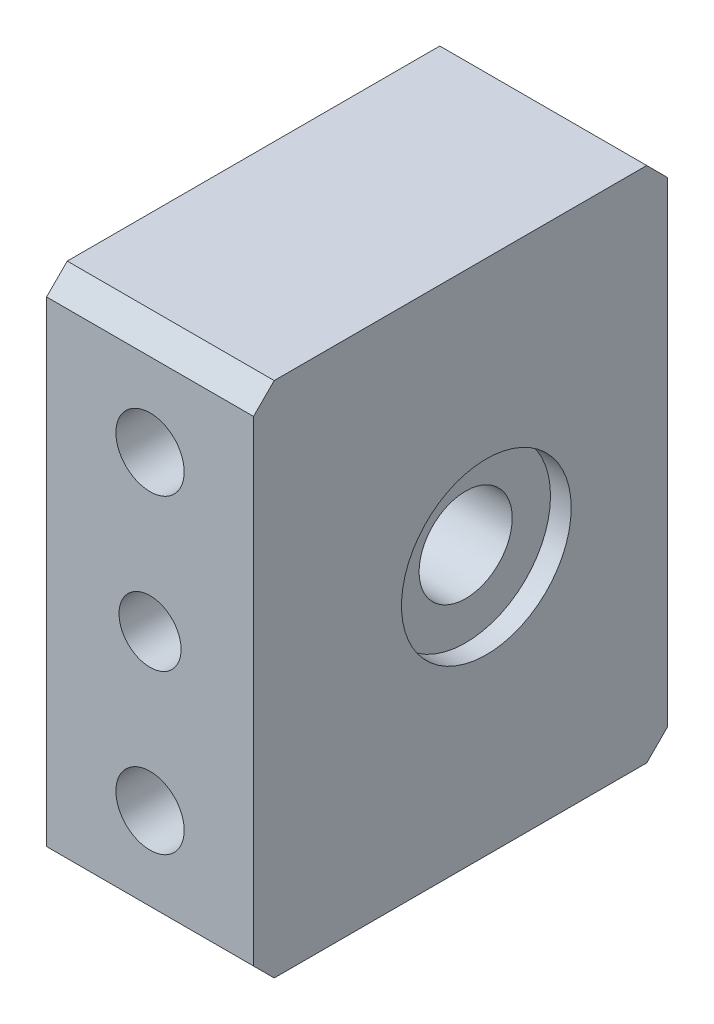
SolidWorks part; units mm, degrees
material "A6061 T6"
ref_plane "前视基准面" through (0, 0, 0) normal (0, 0, 1) x (1, 0, 0)
ref_plane "上视基准面" through (0, 0, 0) normal (0, 1, 0) x (1, 0, 0)
ref_plane "右视基准面" through (0, 0, 0) normal (1, 0, 0) x (0, 0, -1)
sketch "草图1" plane through (0, 0, 0) normal (0, 1, 0) x (1, 0, 0)
  line L1 (-5, 10) -> (5, 10)
  line L2 (-5, 10) -> (-5, -10)
  line L3 (-5, -10) -> (5, -10)
  line L4 (5, 10) -> (5, -10)
  line L5 (-5, 10) -> (5, -10) construction
  line L6 (-5, -10) -> (5, 10) construction
  point P0 (0, 0)
  dimension "D1" = 10
  dimension "D2" = 20
extrude "凸台-拉伸1" add sketch "草图1" along normal blind 25
hole_wizard "打孔尺寸(%根据)内六角圆柱头螺钉的类型1" positions "草图2" profile "草图3" counterbore size "M4" standard "GB"
sketch "草图2" plane through (-5, 0, 0) normal (-1, 0, 0) x (0, 0, 1)
  point P0 (-1.25, 12.5)
sketch "草图3" plane through (-5, 12.5, -1.25) normal (0, 1, 0) x (0, 0, 1)
  line L0 (0, 0) -> (0, 11.4519)
  line L1 (0, 11.4519) -> (2.25, 10.1)
  line L2 (2.25, 10.1) -> (2.25, 4.6)
  line L3 (2.25, 4.6) -> (4, 4.6)
  line L4 (4, 4.6) -> (4, 0)
  line L5 (4, 0) -> (0, 0)
  line L10 (0, 11.4519) -> (-2.25, 10.1) construction
  line L11 (0, -6.35) -> (0, 107.95) construction
  dimension "孔直径" = 4.5
  dimension "孔深度" = 10.1
  dimension "柱形沉头孔直径" = 8
  dimension "柱形沉头孔深度" = 4.6
  dimension "导头角度" = 118
sketch "草图4" plane through (5, 0, 0) normal (1, 0, 0) x (0, 0, -1)
  circle A0 centre (1.25, 12.5) radius 4.1
  dimension "D1" = 8.2
extrude "切除-拉伸1" cut sketch "草图4" against normal blind 1
hole_wizard "M4 螺纹孔1" positions "草图5" profile "草图6" tap size "M4" standard "GB"
sketch "草图5" plane through (0, 0, 10) normal (0, 0, 1) x (1, 0, 0)
  line L0 (-5, 25) -> (5, 25) construction
  line L1 (-5, 0) -> (5, 0) construction
  line L2 (-5, 25) -> (-5, 0) construction
  point P0 (0, 20)
  point P2 (0, 5)
  dimension "D1" = 5
  dimension "D2" = 5
  dimension "D3" = 5
sketch "草图6" plane through (0, 20, 10) normal (1, 0, 0) x (0, -1, 0)
  line L0 (0, 0) -> (0, 11.0914)
  line L1 (0, 11.0914) -> (1.65, 10.1)
  line L2 (1.65, 10.1) -> (1.65, 0)
  line L5 (1.65, 0) -> (0, 0)
  line L10 (0, 11.0914) -> (-1.65, 10.1) construction
  line L11 (0, -6.35) -> (0, 107.95) construction
  dimension "螺纹孔钻头直径" = 3.3
  dimension "螺纹孔钻头深度" = 10.1
  dimension "导头角度" = 118
cosmetic thread "孔螺蚊线1" parameters "D1"=8, "D2"=4
cosmetic thread "孔螺蚊线2" parameters "D1"=8, "D2"=4
hole_wizard "大小mm 暗销孔1" positions "草图7" profile "草图8" hole size "Ø3.0" standard "GB"
sketch "草图7" plane through (0, 0, 10) normal (0, 0, 1) x (1, 0, 0)
  line L0 (-5, 25) -> (5, 25) construction
  line L2 (-5, 25) -> (-5, 0) construction
  point P0 (0, 12.5)
  dimension "D1" = 12.5
  dimension "D2" = 5
sketch "草图8" plane through (0, 12.5, 10) normal (1, 0, 0) x (0, -1, 0)
  line L0 (0, 0) -> (0, 6.9013)
  line L1 (0, 6.9013) -> (1.5, 6)
  line L2 (1.5, 6) -> (1.5, 0)
  line L5 (1.5, 0) -> (0, 0)
  line L10 (0, 6.9013) -> (-1.5, 6) construction
  line L11 (0, -6.35) -> (0, 107.95) construction
  dimension "孔直径" = 3
  dimension "孔深度" = 6
  dimension "导头角度" = 118
chamfer "倒角1" distance 1 angle 45 4 edges at (0, 0, 10) (0, 0, -10) (0, 25, -10) (0, 25, 10)
